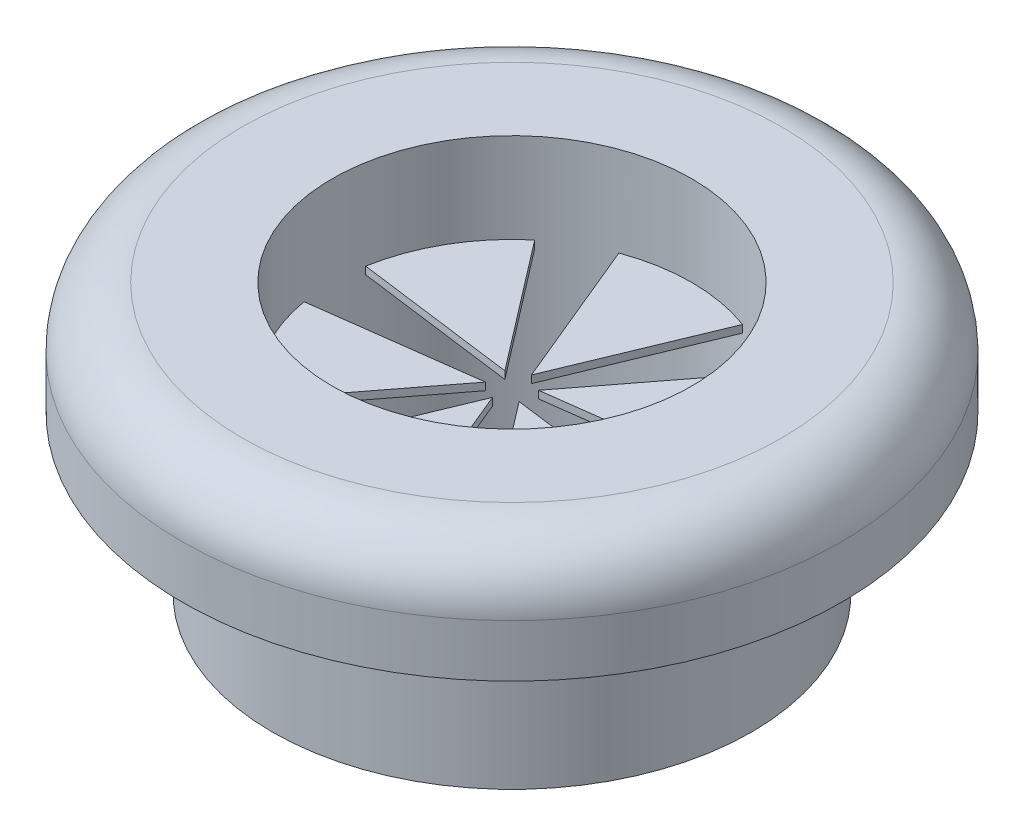
SolidWorks part; units mm, degrees
ref_plane "Front Plane" through (0, 0, 0) normal (0, 0, 1) x (1, 0, 0)
ref_plane "Top Plane" through (0, 0, 0) normal (0, 1, 0) x (1, 0, 0)
ref_plane "Right Plane" through (0, 0, 0) normal (1, 0, 0) x (0, 0, -1)
sketch "Sketch1" plane through (0, 0, 0) normal (0, 1, 0) x (1, 0, 0)
  circle A0 centre (0, 0) radius 8
  dimension "D1" = 16
extrude "Boss-Extrude1" add sketch "Sketch1" along normal blind 5
sketch "Sketch2" plane through (0, 5, 0) normal (0, 1, 0) x (1, 0, 0)
  circle A0 centre (0, 0) radius 11
  dimension "D1" = 22
extrude "Boss-Extrude2" add sketch "Sketch2" along normal blind 4
sketch "Sketch3" plane through (0, 9, 0) normal (0, 1, 0) x (1, 0, 0)
  circle A0 centre (0, 0) radius 6
  dimension "D1" = 12
extrude "Cut-Extrude1" cut sketch "Sketch3" against normal up to next
sketch "Sketch4" plane through (0, 0, 0) normal (0, -1, 0) x (1, 0, 0)
  line L0 (0, 0) -> (0, 6) construction
  line L1 (0, 0.65) -> (-2.0643, 5.6337)
  line L2 (0, 0.65) -> (2.0643, 5.6337)
  line L3 (0.5629, 0.325) -> (3.8468, 4.6046)
  line L4 (0, 0) -> (5.1962, 3) construction
  line L5 (0.5629, 0.325) -> (5.9111, 1.0291)
  line L6 (0.5629, -0.325) -> (5.9111, -1.0291)
  line L7 (0, 0) -> (5.1962, -3) construction
  line L8 (0.5629, -0.325) -> (3.8468, -4.6046)
  line L9 (0, -0.65) -> (2.0643, -5.6337)
  line L10 (0, 0) -> (0, -6) construction
  line L11 (0, -0.65) -> (-2.0643, -5.6337)
  line L12 (-0.5629, -0.325) -> (-3.8468, -4.6046)
  line L13 (0, 0) -> (-5.1962, -3) construction
  line L14 (-0.5629, -0.325) -> (-5.9111, -1.0291)
  line L15 (-0.5629, 0.325) -> (-5.9111, 1.0291)
  line L16 (0, 0) -> (-5.1962, 3) construction
  line L17 (-0.5629, 0.325) -> (-3.8468, 4.6046)
  circle A0 centre (0, 0) radius 6 construction
  arc A1 (-2.0643, 5.6337) -> (2.0643, 5.6337) centre (0, 0) cw
  arc A2 (3.8468, 4.6046) -> (5.9111, 1.0291) centre (0, 0) cw
  arc A3 (5.9111, -1.0291) -> (3.8468, -4.6046) centre (0, 0) cw
  arc A4 (2.0643, -5.6337) -> (-2.0643, -5.6337) centre (0, 0) cw
  arc A5 (-3.8468, -4.6046) -> (-5.9111, -1.0291) centre (0, 0) cw
  arc A6 (-5.9111, 1.0291) -> (-3.8468, 4.6046) centre (0, 0) cw
  point P31 (0, 0)
  dimension "D1" = 0.65
  dimension "D2" = 45
  dimension "D3" = 6
extrude "Boss-Extrude3" add sketch "Sketch4" along normal blind 0.25 from offset 6 offset against normal yes
sketch "Sketch5" plane through (0, 5, 0) normal (0, -1, 0) x (1, 0, 0)
  circle A0 centre (0, 0) radius 10
  circle A1 centre (0, 0) radius 11
  circle A2 centre (0, 0) radius 11
  dimension "D1" = 0
  dimension "D2" = 1
extrude "Cut-Extrude2" cut sketch "Sketch5" against normal blind 0.25
fillet "Fillet1" radius 2 1 edges at (0, 9, 11)
